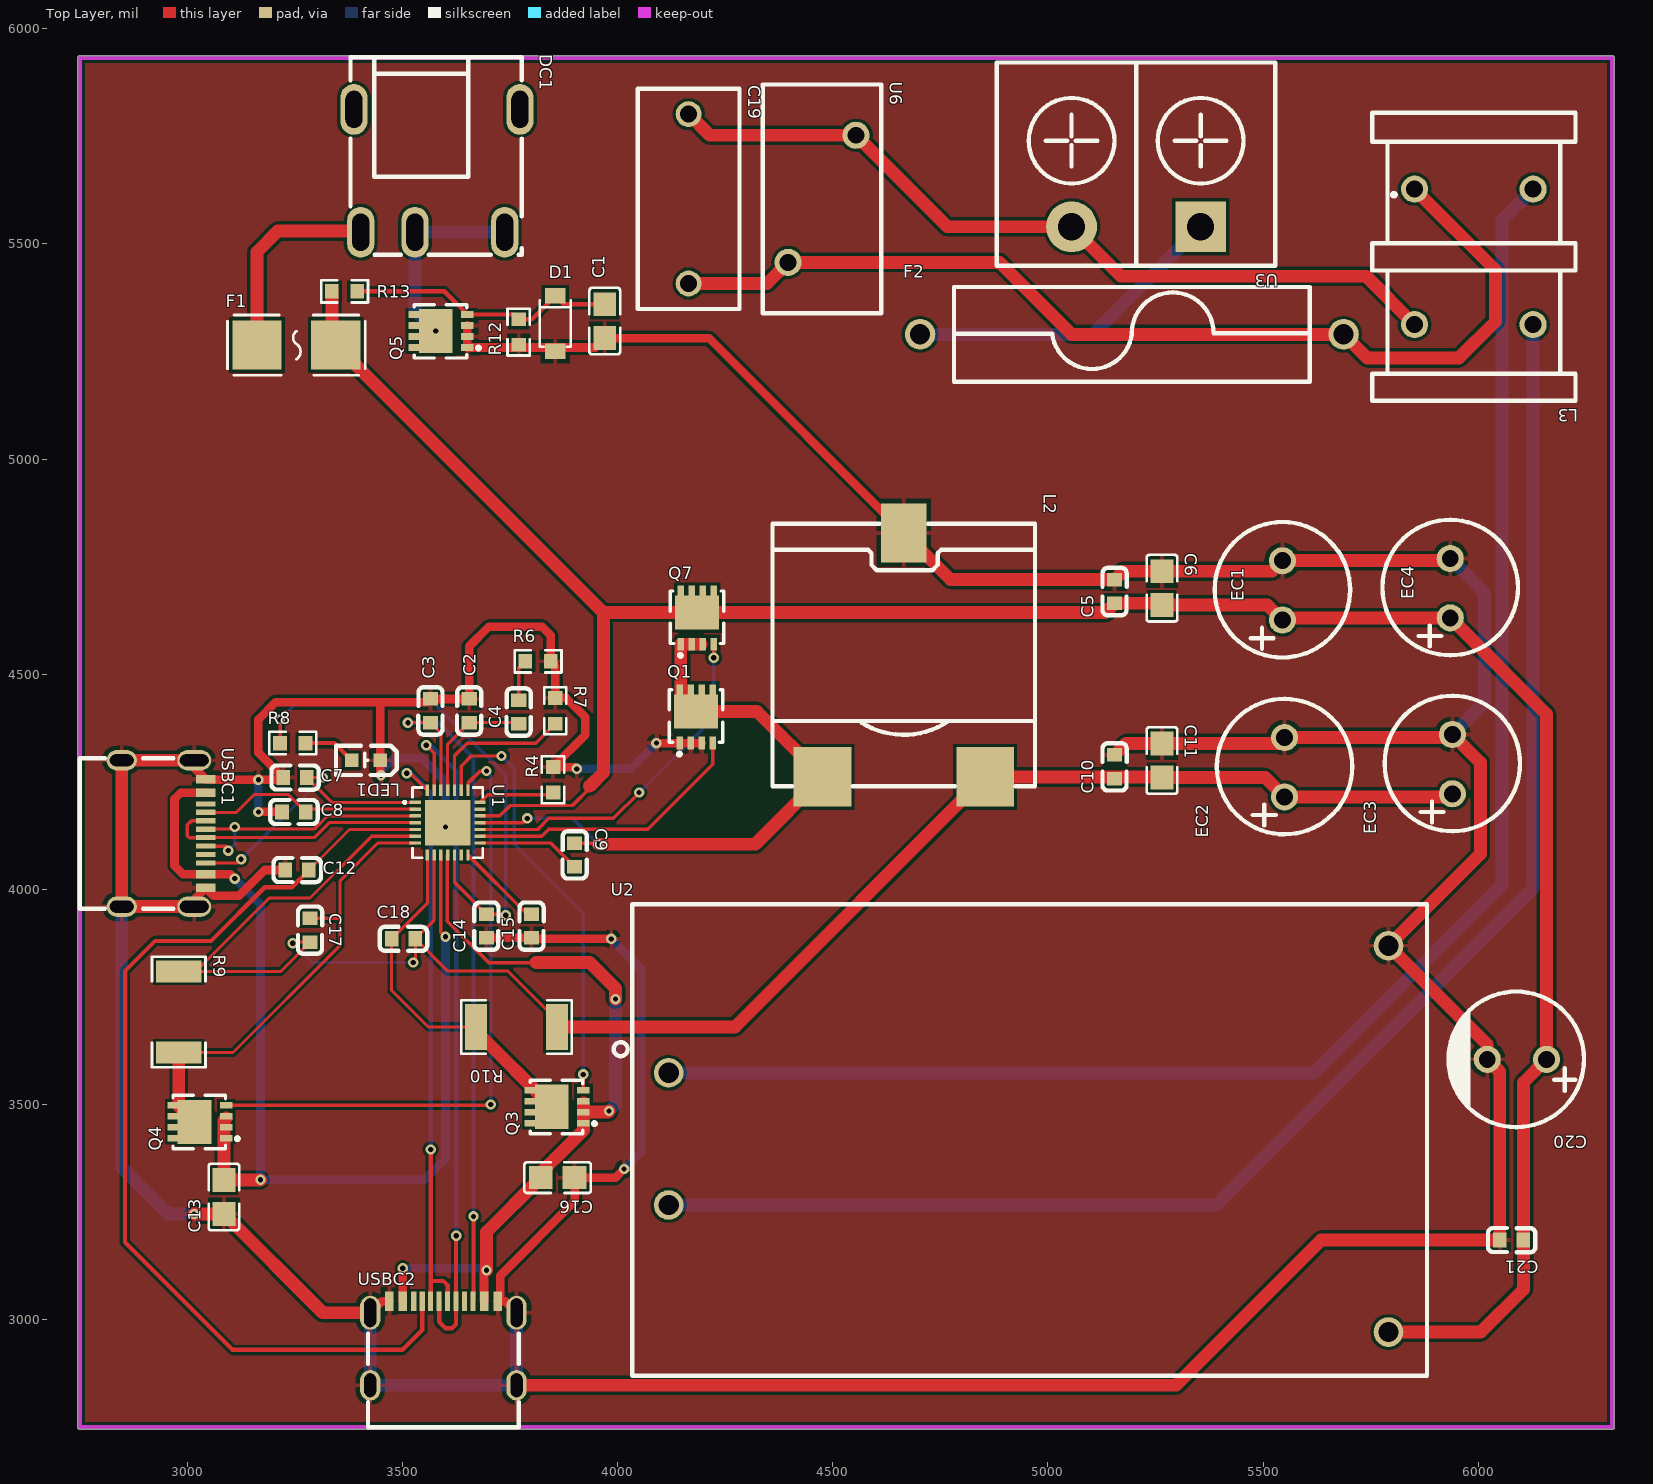
[diagram p0: Top Layer view]
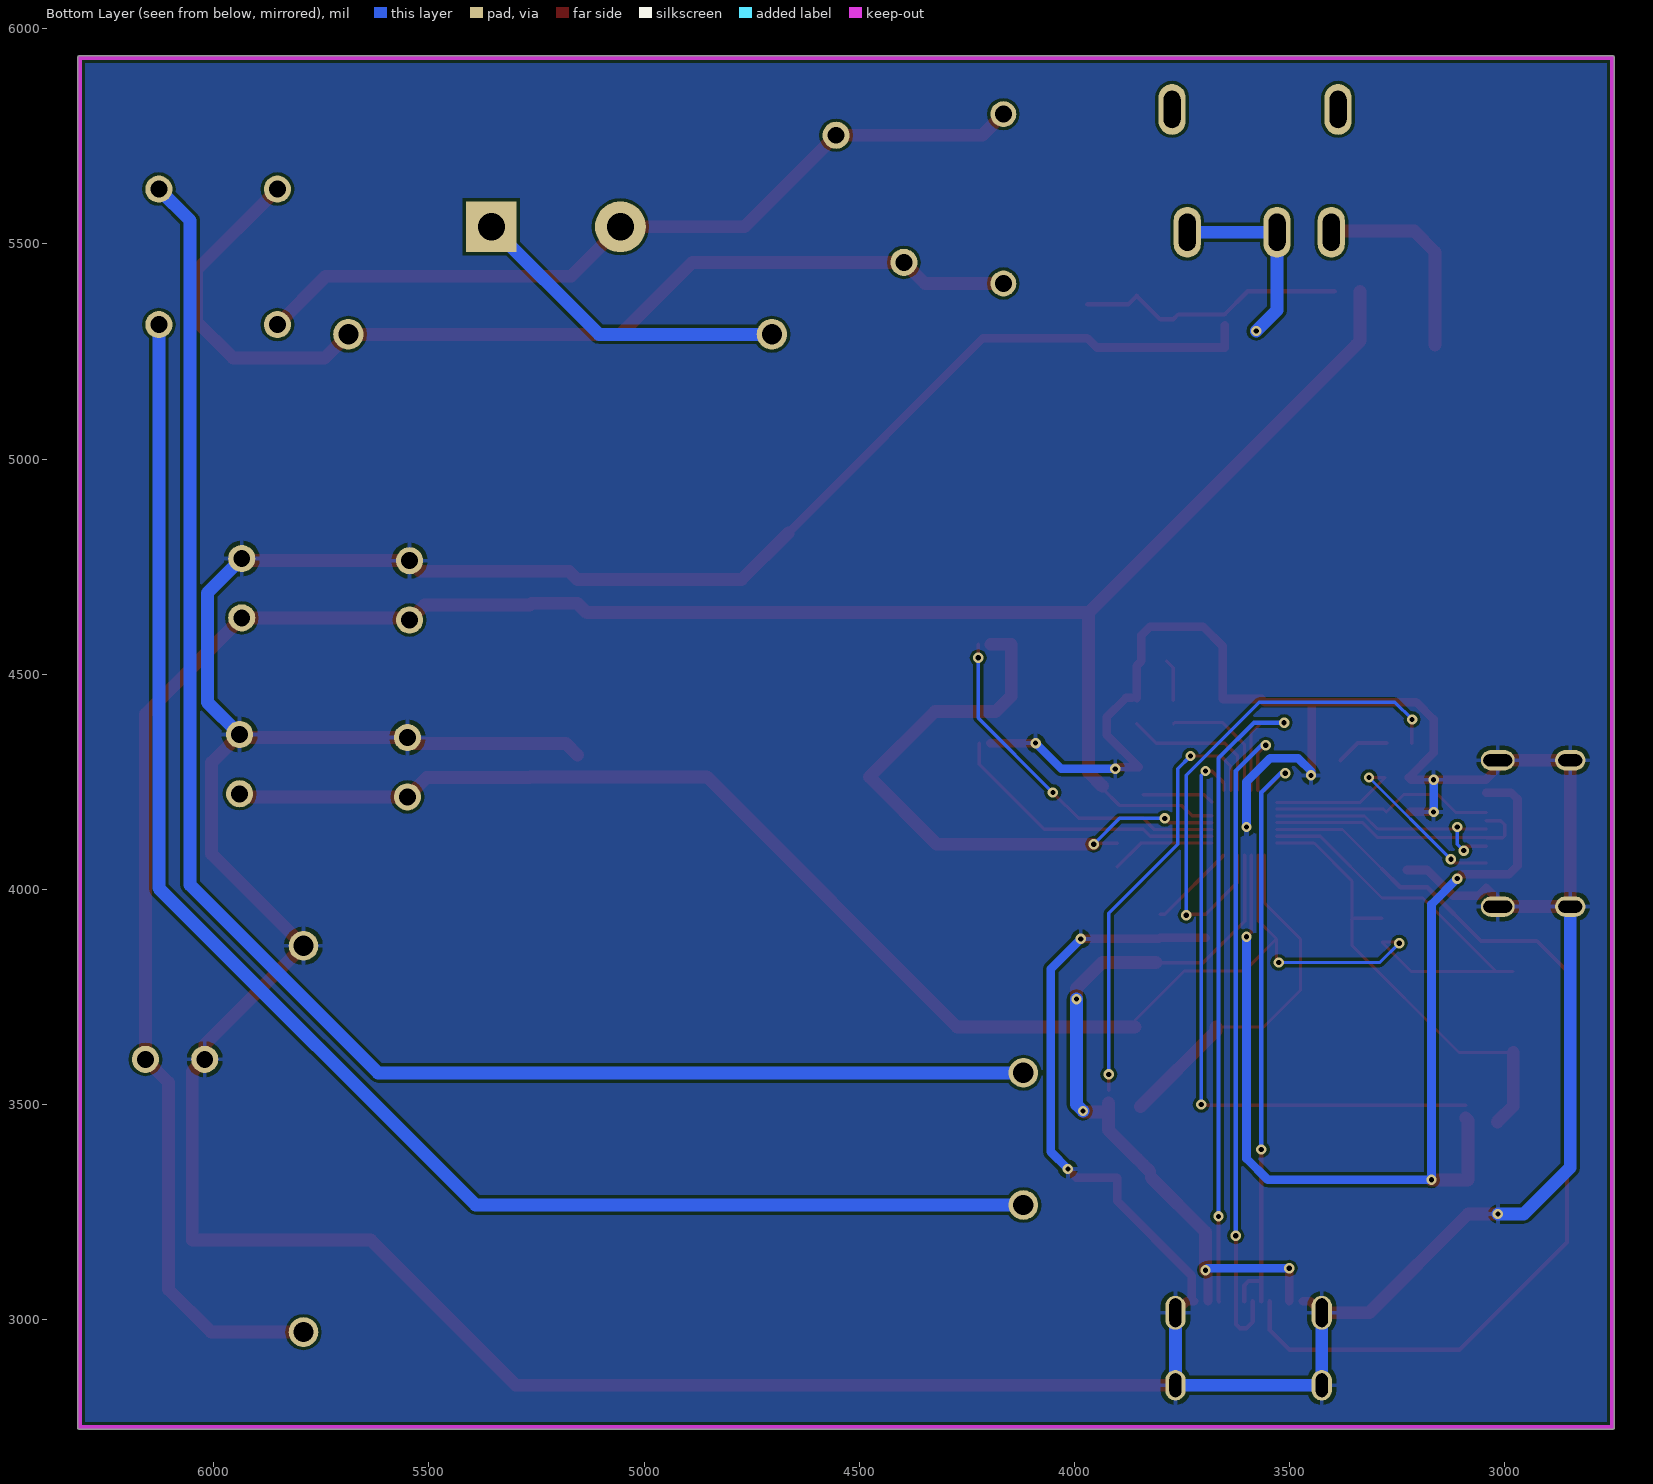
[diagram p1: Bottom Layer view, seen from below]
# Altium PCB MISC82101.pcbdoc
Units mil, origin at the board's own origin, x right, y up, seen from the top; angles counter-clockwise.
Board outline 3571.45 x 3192.71 mil, 2 copper layers (Top Layer, Bottom Layer); 51 components, 36 nets, 208 pads, 39 vias.

## Layer stack, top to bottom (the 12.6 mil dielectric is the usual default, probably not edited)
Top Solder Mask Layer: solder mask 0.4, Solder Resist, Dk 3.5
Top Layer: signal copper 1.4
Dielectric1: dielectric 12.6, FR-4, Dk 4.8
Bottom Layer: signal copper 1.4
Bottom Solder Mask Layer: solder mask 0.4, Solder Resist, Dk 3.5

## Board outline
2750,2744.99 cw(c2750,2750) 2744.99,2750 2744.99,5932.68 cw(c2750,5932.68) 2750,5937.69 6309.09,5937.69 cw(c6309.09,5932.68) 6310.26,5937.56 cw(c6311.42,5932.68) 6316.43,5932.68 6316.43,2750 cw(c6311.42,2750) 6311.42,2744.99

## Design rules (kind name [scope] priority, off if disabled: settings)
Clearance [All] p1: gap=7
MinimumSolderMaskSliver [All] p1: minsoldermaskwidth=0
PolygonConnect [All] p1: connectstyle=Relief reliefconductorwidth=10 reliefentries=4 polygonreliefangle="90 Angle" airgapwidth=10
RoutingVias [All] p1: holewidth=28 width=50 viastyle="Through Hole" minholewidth=28 minwidth=50 maxholewidth=28 maxwidth=50
SilkToSilkClearance [All] p1: silktosilkclearance=0
SilkToSolderMaskClearance [IsPad] p1: minsilkscreentomaskgap=0 clearancetoexposedcopper=TRUE
SolderMaskExpansion [All] p1: expansion=4
Width [All] p1: maxlimit=50 minlimit=7 preferedwidth=10 minimp=50.000000 maximp=50.000000 favimp=50.000000
27 further rules are at their usual default settings.

## Components (designator, comment, footprint, x,y, rotation, side; value= is the part's Value field where it differs from the comment)
C1 "10uF" C0805 3970,5320.63 r90 top
C2 "100pF" C0603 3655,4415 r90 top
C3 "330pF" C0603 3565,4415 r90 top
C4 "2.2nF" C0603 3770,4412.44 r90 top
C5 "100nF" C0603 5155,4692.56 r90 top
C6 "10uF" C0805 5265,4700 r270 top
C7 "330pF" C0603 3250,4260 r180 top
C8 "330pF" C0603 3247.44,4180 r180 top
C9 "100nF" C0603 3900,4080 r270 top
C10 "100nF" C0603 5155,4285 r90 top
C11 "22uF" C0805 5265,4299.37 r270 top
C12 "330pF" C0603 3255,4045 r180 top
C13 "10uF" C0805 3085,3285 r90 top
C14 "1uF" C0603 3695,3915 r90 top
C15 "1uF" C0603 3800,3915 r90 top
C16 "10uF" C0805 3860.63,3330 r180 top
C17 "100nF" C0603 3285,3905 r270 top
C18 "100nF" C0603 3502.44,3885 r0 top
C19 "100nF" CAP-TH_L13.0-W6.0-P10.0-D0.6 4165,5605 r270 top
C20 "220uF" CAP-TH_BD8.0-P3.50-D0.6-FD 6090,3605 r180 top
C21 "100nF" C0603 6077.56,3185 r180 top
D1 "BZT52C3V3" SOD-123_L2.7-W1.6-LS3.7-RD 3855,5315 r270 top
DC1 "DC-044A-20A" DC-IN-TH_DC-044A-20A 3580,5670 r270 top
EC1 "220uF" CAP-TH_BD8.0-P3.50-D0.6-FD-2 5545,4695 r90 top
EC2 "220uF" CAP-TH_BD8.0-P3.50-D0.6-FD-2 5550,4283.9 r90 top
EC3 "220uF" CAP-TH_BD8.0-P3.50-D0.6-FD-2 5940,4291.1 r90 top
EC4 "220uF" CAP-TH_BD8.0-P3.50-D0.6-FD-2 5935,4700 r90 top
F1 "0451008.MRL" FUSE-SMD_L6.1-W2.7 3253.3,5265 r0 top
F2 "5G.0015222000S1(5)" FUSE-TH_BD5.6-L21.0-P25.00-D0.7 5195,5290 r0 top
L2 "22uH" IND-SMD_3P-L15.5-W15.5-L 4665,4545 r270 top
L3 "UU9.8-20mH" FILTER-TH_4P-L17.0-W12.0-P7.00-D0.6-S8.00 5990,5470 r180 top
LED1 "19-217/BHC-ZL1M2RY/3T" LED0603-R-RD 3415,4300 r180 top
Q1 "RUH4040M2" PDFN3333-8_L3.1-W3.2-P0.65-LS3.4-BL 4182.79,4400.37 r0 top
Q3 "RUH4040M2" PDFN3333-8_L3.1-W3.2-P0.65-LS3.4-BL 3860,3495 r90 top
Q4 "RUH4040M2" PDFN3333-8_L3.1-W3.2-P0.65-LS3.4-BL 3030,3460 r90 top
Q5 "RUH4040M2" PDFN3333-8_L3.1-W3.2-P0.65-LS3.4-BL 3590.37,5297.79 r90 top
Q7 "RUH4040M2" PDFN3333-8_L3.1-W3.2-P0.65-LS3.4-BL 4185,4630 r0 top
R4 "Rpset" R0603 3850,4254.66 r270 top
R6 "20kΩ" R0603 3815,4530 r0 top
R7 "SDNT1608X104F4250FTF" R0603 3855,4415 r270 top
R8 "0603WAF2001T5E" R0603 3245,4340 r0 top
R9 "RLM20FECR005" R2010 2980,3715 r270 top
R10 "RLM20FECR005" R2010 3765,3680 r180 top
R12 "10kΩ" R0603 3770,5295.34 r90 top
R13 "0603WAF5102T5E" R0603 3365.34,5390 r180 top
U1 "sw3556-1" QFN-28_L4.0-W4.0-P0.40-BL-EP 3605,4155 r270 top
U2 "HLK-10M24" PWRM-TH_HLK-10M24 4955,3420 r0 top
U3 "KF7.62-2P" CONN-TH_KF7.62-2P 5205,5540 r180 top
U6 "10D561K68RV0095" RES-TH_L13.5-W7.0-P7.50-S4.00-D0.7 4475,5605 r270 top
USBC1 "U263-163N-4OS1735" USB-C-SMD_U263-163N-4GS1735 2945,4130 r270 top
USBC2 "U263-163N-4OS1735" USB-C-SMD_U263-163N-4GS1735 3595,2945 r0 top

## Footprints (in the part's own frame and the unit in brackets; to place one, negate y for a bottom-side part, rotate by r counter-clockwise, add the part's x,y. Pads: shape width x height; smd on the part's side, far side on the other; paste and mask are expansions set on the pad)
C0603 [mm]
  rect 0.8x0.9 smd paste+0 mask+0.051: 1(-0.7,0) 2(0.7,0)
  silkscreen extent -1.41,-0.71 1.39,0.72
C0805 [mm]
  rect 1.41x1.35 smd paste-100 mask+0.051: 1(-1,0) 2(1,0)
  silkscreen extent -1.96,-0.9 1.96,0.9
CAP-TH_BD8.0-P3.50-D0.6-FD [mm]
  round 1.6 hole 1: 1(-1.75,0) 2(1.75,0)
  silkscreen extent -3.96,-4 4.04,4
CAP-TH_BD8.0-P3.50-D0.6-FD-2 [mm]
  round 1.6 hole 1 paste+0 mask+0.051: 1(-1.75,0) 2(1.75,0)
  silkscreen extent -3.96,-4 4.04,4
CAP-TH_L13.0-W6.0-P10.0-D0.6 [mil]
  round 60 hole 39.37: 1(-196.85,0) 2(196.85,0)
  silkscreen extent -256,-118 256,118
CONN-TH_KF7.62-2P [mm]
  rect 3x3 hole 1.6: 1(-3.81,0)
  round 3 hole 1.6: 2(3.81,0)
  silkscreen extent -8.22,-9.7 8.22,2.3
DC-IN-TH_DC-044A-20A [mm]
  oval 3x1.6 hole 1 slot 2.2 at 0 deg paste+0 mask+0.051: 1(3.625,-4.5) 2(3.625,4.001) 3(3.625,-1.3) 4(-3.625,-4.9) 5(-3.625,4.9)
  silkscreen extent -6.7,-5.1 4.95,5
FILTER-TH_4P-L17.0-W12.0-P7.00-D0.6-S8.00 [mm]
  round 1.6 hole 1: 1(3.5,-4) 2(-3.5,-4) 3(-3.5,4) 4(3.5,4)
  silkscreen extent -6,-8.5 6,8.5
FUSE-SMD_L6.1-W2.7 [mil]
  rect 114.6x114.4 smd paste-3937.01 mask+2: 1(-91.7,0) 2(91.7,0)
  silkscreen extent -160,-70 160,70
FUSE-TH_BD5.6-L21.0-P25.00-D0.7 [mm]
  round 1.8 hole 1.2: 1(-12.5,0) 2(12.5,0)
  silkscreen extent -10.5,-2.8 10.5,2.8
IND-SMD_3P-L15.5-W15.5-L [mil]
  rect 137.8x106.3 smd paste+0 mask+2: 1(-283.5,0)
  rect 137.8x133.9 smd paste+0 mask+2: 2(283.5,-189) 3(283.5,189)
  silkscreen extent -305,-305 305,305
LED0603-R-RD [mm]
  rect 0.8x0.8 smd paste+0 mask+0.051: 1(0.851,0) 2(-0.851,0)
  silkscreen extent -1.82,-0.86 1.77,0.86
PDFN3333-8_L3.1-W3.2-P0.65-LS3.4-BL [mm]
  rect 0.4x0.75 smd paste-100 mask+0.051: 1(-0.975,-1.533) 2(-0.325,-1.533) 3(0.325,-1.533) 4(0.975,-1.533)
  rect 0.4x0.8 smd paste-100 mask+0.051: 5(0.975,1.533) 6(0.325,1.533) 7(-0.325,1.533) 8(-0.975,1.533)
  rect 2.6x2 smd paste-100 mask+0.051: 9(-0.005,0.333)
  silkscreen extent -1.59,-2.29 1.56,1.61
PWRM-TH_HLK-10M24 [mm]
  round 1.75 hole 1.2 paste+0 mask+0.05: 1(-21.25,3.9) 2(-21.25,-3.9) 3(21.25,11.4)
  round 1.75 hole 1.2 copper offset 0,0 paste+0 mask+0.05: 4(21.25,-11.4)
  silkscreen extent -24.49,-13.98 23.52,13.86
QFN-28_L4.0-W4.0-P0.40-BL-EP [mm]
  rect 0.2x0.665 smd paste-100 mask+0.051: 1(-1.2,-1.908) 2(-0.8,-1.908) 3(-0.4,-1.908) 4(0,-1.908) 5(0.4,-1.908) 6(0.8,-1.908) 7(1.2,-1.908) 15(1.2,1.908) 16(0.8,1.908) 17(0.4,1.908) 18(0,1.908) 19(-0.4,1.908) 20(-0.8,1.908) 21(-1.2,1.908)
  rect 0.665x0.2 smd paste-100 mask+0.051: 8(1.908,-1.2) 9(1.908,-0.8) 10(1.908,-0.4) 11(1.908,0) 12(1.908,0.4) 13(1.908,0.8) 14(1.908,1.2) 22(-1.908,1.2) 23(-1.908,0.8) 24(-1.908,0.4) 25(-1.908,0) 26(-1.908,-0.4) 27(-1.908,-0.8) 28(-1.908,-1.2)
  rect 2.7x2.7 smd paste-100 mask+0.051: 29(0,0)
  silkscreen extent -2.08,-2.61 2.08,2.08
R0603 [mil]
  rect 31.75x34.02 smd paste-3937.01 mask+2: 1(-29.66,0) 2(29.66,0)
  silkscreen extent -55,-26 55,26
R2010 [mm]
  rect 1.283x2.7 smd paste-100 mask+0.051: 1(-2.391,0) 2(2.391,0)
  silkscreen extent -3.26,-1.58 3.26,1.58
RES-TH_L13.5-W7.0-P7.50-S4.00-D0.7 [mm]
  round 1.6 hole 1 paste+0 mask+0.05: 1(-3.75,2) 2(3.75,-2)
  silkscreen extent -6.75,-3.5 6.75,3.5
SOD-123_L2.7-W1.6-LS3.7-RD [mm]
  rect 0.91x1.22 smd paste+0 mask+0.051: 1(-1.635,0) 2(1.635,0)
  silkscreen extent -1.38,-0.93 1.38,0.93
USB-C-SMD_U263-163N-4GS1735 [mm]
  rect 0.5x1.15 smd paste-100 mask+0.051: A1(-3.2,2.478) A4(-2.4,2.478) A9(2.4,2.478) A12(3.218,2.478) B1(3.218,2.478) B4(2.4,2.478) B9(-2.4,2.478) B12(-3.2,2.478)
  rect 0.3x1.15 smd paste-100 mask+0.051: A5(-1.25,2.478) A6(-0.25,2.478) A7(0.25,2.478) A8(1.25,2.478) B5(1.75,2.478) B6(0.75,2.478) B7(-0.75,2.478) B8(-1.75,2.478)
  oval 1.2x1.8 hole 0.7 slot 1.4 at 90 deg paste+0 mask+0.051: SH1(-4.32,-2.477) SH1(4.32,-2.477)
  oval 1.2x2 hole 0.7 slot 1.7 at 90 deg copper offset 0,0 paste+0 mask+0.051: SH1(-4.32,1.802)
  oval 1.2x2 hole 0.7 slot 1.7 at 90 deg paste+0 mask+0.051: SH1(4.32,1.802)
  silkscreen extent -4.44,-4.96 4.45,0.58

## Part data
C1 C6 C13 C16: "Capacitance: 10uF; tolerance: ±10%; rated voltage: 50V; dielectric (temperature coefficient): X5R;"
C2: "Capacitance: 100pF; tolerance: ±5%; rated voltage: 50V; dielectric (temperature coefficient): C0G;"
C3 C7 C8 C12: "Capacitance: 330pF; tolerance: ±5%; rated voltage: 50V; dielectric (temperature coefficient): C0G;"
C4: "Capacitance: 2.2nF; tolerance: ±1%; rated voltage: -; dielectric (temperature coefficient): -;"
C5 C9 C10 C17 C18 C21: "Capacitance: 100nF; tolerance: ±10%; rated voltage: 50V; dielectric (temperature coefficient): X7R;"
C11: "Capacitance: 22uF; tolerance: ±20%; rated voltage: 25V; dielectric (temperature coefficient): X5R;"
C14 C15: "Capacitance: 1uF; tolerance: ±10%; rated voltage: 50V; dielectric (temperature coefficient): X5R;"
C19: library part X2-104K-275VAC_C914483
C20: library part 01EC3470
D1: "Diode configuration: single; zener voltage (nominal): 3.3V; zener voltage (range): 3.1V~3.5V; tolerance: ±5%; power: 500mW; reverse current (Ir): 20uA@1V; impedance (Zzt): 130Ω;"
DC1: "Contact inner diameter: 2mm; contact outer diameter: 5.9mm; rated current: 500mA; rated voltage: 30V;"
EC1 EC2 EC3 EC4: "容值:220uF;精度:±20%;额定电压:35V;电容体直径:8mm;电容体长度:9mm;脚间距:3.5mm;纹波电流:1.7A@100kHz;等效串联电阻:40mΩ@100kHz;工作寿命:2000hrs@105℃;工作温度:-55℃~+105℃;"
F1: "Type: SMD fuse; rated current: 8A; rated voltage (AC): 125V; rated voltage (DC): 125V; breaking capacity: 50A; operating temperature: -55℃~+125℃;"
L2: "Inductance: 22uH; tolerance: ±20%; rated current: 7.5A; DC resistance (DCR): 14.5mΩ;"
LED1: "Illumination color: blue; dominant wavelength / chromaticity: 465~475nm;"
Q1 Q3 Q4 Q5 Q7: "类型:-;漏源电压(Vdss):-;连续漏极电流(Id):-;功率(Pd):-;导通电阻(RDS(on)@Vgs,Id):-;阈值电压(Vgs(th)@Id):-;栅极电荷(Qg@Vgs):-;输入电容(Ciss@Vds):-;反向传输电容(Crss@Vds):-;"
R4: "Resistor"
R6: "Tolerance: ±1%; temperature coefficient: ±100ppm/℃; resistance: 20kΩ; power: 1/10W; max working voltage: 75V; operating temperature range: -55℃~+155℃;"
R7: "阻值(25℃):100kΩ;电阻精度:±1%;B值精度:±1%;B值(25℃/50℃):4250K;功率:100mW;最大稳态电流(25℃):100uA;B值(25℃/75℃):-;B值(25℃/85℃):-;B值(25℃/100℃):-;工作温度:-55℃~+125℃;"
R8: "Tolerance: ±1%; resistance: 2kΩ; temperature coefficient: ±100ppm/℃; power: 1/10W; max working voltage: 75V; operating temperature range: -55℃~+155℃;"
R9 R10: "Resistor type: sense resistor; rated current: -; rated voltage drop: -; resistance: 5mΩ; tolerance: ±1%; power: 1W; temperature coefficient: ±50ppm/℃; mounting: SMD;"
R12: "Resistor type: thick film; resistance: 10kΩ; tolerance: ±1%; power: 100mW; temperature coefficient: ±100ppm/℃; max working voltage: 75V; operating temperature range: -55℃~+155℃;"
USBC1 USBC2: "连接器类型:Type-C;标准:USB 3.1;公母:母座;触点数量:16;端口数量:1;安装方式:卧贴;额定电流 - 电源:5A;触头材质:铜合金;触头镀层:金;工作温度范围:-25℃~+85℃;焊接温度(最大值):260℃;"

## Via types
v1: diameter 24, hole 12, Top Layer to Bottom Layer, 39 vias

## Nets (pads, with @x,y where several pads share a name; then routed paths per layer and width w, separated by ;. In a path a pad name is that pad's centre, name@x,y a point inside that pad or via, vN(x,y) a via of type N, cw(c..) or ccw(c..) an arc to the next point about the centre after c; other vN are vias at no path point)
BST: C9.2 U1.15 | length 242.8
  Top Layer w8: U1.15 3844.68,4107.76 C9.2
CC11: C8.1 U1.2 USBC1.A5 | length 523.5
  Top Layer w7: USBC1.A5 3114.21,4179.21 3155,4220 3235,4220 C8.1 3281.5,4186.5 U1.2
CC12: C12.1 U1.5 USBC2.A5 | length 2321.3
  Top Layer w7: C12.1@3285,4047.44 3376.81,4139.25 U1.5
  Top Layer w10: C12.1@3285,4047.44 C12.1 3242.56,4005 3180,4005 3055,3880 2925,3880 2855,3810 2855,3180 3105,2930 3500,2930 3545.79,2975.79 USBC2.A5
CC21: C7.1 U1.1 USBC1.B5 | length 668.6
  Top Layer w7: USBC1.B5 3116.1,4061.1 v1(3125,4070) ; v1(3315,4260) C7.1 3335.32,4202.24 U1.1
  Bottom Layer w7: v1(3125,4070) v1(3315,4260)
CC22: C3.1 U1.26 USBC2.B5 | length 1673
  Top Layer w7: v1@3510,4385 v1(3512.44,4387.44) C3.1 3589.25,4363.19 U1.26
  Top Layer w10: USBC2.B5 3665,3043.64 v1(3665,3240)
  Bottom Layer w10: v1(3512.44,4387.44) 3582.56,4387.44 3665,4305 v1(3665,3240)
COMP: C2.1 C4.1 U1.25 | length 294.1
  Top Layer w7: U1.25 3605,4337.44 C2.1 3767.44,4387.44 C4.1
CSN1: C17.1 Q4.5 Q4.6 Q4.7 Q4.8 Q4.9 R9.2 U1.7 | length 1086.8
  Top Layer w7: R9.2 3105.86,3620.86 3355,3870 3355,3930 3355,4020 3442.76,4107.76 U1.7
  Top Layer w8: C17.1 3352.44,3932.56 3355,3930
  Top Layer w30: R9.2 2980,3496.71 Q4.9
CSN2: C18.1 Q3.5 Q3.6 Q3.7 Q3.8 Q3.9 R10.2 U1.8 | length 838.4
  Top Layer w7: U1.8 3557.76,3967.88 C18.1 3474.88,3765.12 3560,3680 R10.2
  Top Layer w30: R10.2 3670.86,3670.85 Q3.9
CSP1: C10.1 C11.2 C17.2 C18.2 EC2.1 EC3.1 L2.3 R9.1 R10.1 U1.6 U1.9 | length 4351.2
  Top Layer w7: R9.1 R9.1@3019.14,3809.14 ; v1(3245,3875) 3247.44,3877.44 C17.2 3216.7,3809.14 R9.1@3019.14,3809.14 ; v1(3525,3830) 3530,3835 C18.2 ; U1.6 3428.5,4123.5 3285,3980 3190,3980 R9.1@3019.14,3809.14 ; U1.9 3573.5,3928.5 C18.2 ; R10.1 3859.14,3695.86 3745,3810 3605,3810 C18.2
  Top Layer w30: R10.1 4272.5,3680 L2.3 5263.5,4261.5 C11.2 5505,4260 EC2.1 5932.8,4215 EC3.1
  Bottom Layer w7: v1(3245,3875) 3290,3830 v1(3525,3830)
DM1: U1.4 USBC1.A7 USBC1.B7 | length 618
  Top Layer w7: USBC1.A7 3294.95,4120.15 3329.8,4155 U1.4
  Top Layer w8: USBC1.A7 3005.15,4120.15 3005,4120 3000,4125 3000,4150 3009.52,4159.52 USBC1.B7
DM2: U1.28 USBC2.A7 USBC2.B7 | length 1402.2
  Top Layer w8: v1(3510,4270) 3517.86,4270 U1.28
  Top Layer w10: USBC2.B7 3565.48,3090 ; v1(3565.48,3395.48) 3565.48,3090 ; USBC2.A7 3604.85,3080.15 3595,3090 3565.48,3090
  Bottom Layer w10: v1(3510,4270) 3520.96,4270 3565.48,4225.48 v1(3565.48,3395.48)
DP1: U1.3 USBC1.A6 USBC1.B6 | length 613.4
  Top Layer w7: USBC1.A6 3294.84,4139.84 3325.75,4170.75 U1.3
  Top Layer w8: USBC1.B6 v1@3089.53,4100.47 ; v1@3095,4085 v1(3095,4090)
  Bottom Layer w8: v1(3095,4090) 3110,4105 v1(3110,4145)
DP2: U1.27 USBC2.A6 USBC2.B6 | length 1590.2
  Top Layer w8: v1(3555,4335) 3573.5,4316.5 U1.27
  Top Layer w10: USBC2.A6 3585.16,2994.84 3600,2980 3615,2980 3624.53,2989.53 USBC2.B6 3624.53,3194.53 v1(3625,3195)
  Bottom Layer w10: v1(3555,4335) 3565,4335 3625,4275 v1(3625,3195)
GATE1: Q4.4 U1.22 | length 1465.8
  Top Layer w8: Q4.4 3703.39,3498.39 v1(3705,3500) ; U1.22 3652.24,4247.24 3680,4275 v1(3695,4275)
  Bottom Layer w8: v1(3695,4275) 3705,4265 v1(3705,3500)
GATE2: Q3.4 U1.23 | length 1015.1
  Top Layer w8: U1.23 3636.5,4286.5 3660,4310 v1(3730,4310) ; v1(3920,3570) 3920.37,3569.63 Q3.4
  Bottom Layer w8: v1(3730,4310) 3760,4280 3760,4105 3920,3945 v1(3920,3570)
GND: C1.1 C2.2 C3.2 C5.2 C6.1 C7.2 C8.2 C10.2 C11.1 C12.2 C13.1 C14.1 C15.1 C16.1 C20.2 C21.2 D1.2 EC1.2 EC2.2 EC3.2 EC4.2 L2.1 LED1.2 Q1.1 Q1.2 Q1.3 Q5.1 Q5.2 Q5.3 R4.1 R6.2 R7.1 R12.1 U1.29 U2.3 USBC1.A1 USBC1.A12 USBC1.B1 USBC1.B12 USBC1.SH1 USBC2.A1 USBC2.A12 USBC2.B1 USBC2.B12 USBC2.SH1 | length 14705.9
  Top Layer w20: USBC1.SH1@3015.96,3959.92 3015.96,3976.7 USBC1.B1 3060.83,3985 3120,3985 3180,4045 C12.2 ; USBC1.SH1@3015.96,4300.07 3015.96,4282.57 USBC1.B12 3043.52,4255 v1(3165,4255) 3217.44,4255 C7.2 3165,4317.44 3165,4395 3205,4435 3450,4435 ; v1(3165,4180) C8.2 ; USBC2.SH1@3424.93,3015.96 3451.51,3042.54 USBC2.B12 ; v1(3450,4265) 3448.5,4266.5 LED1.2 3448.5,4433.5 3450,4435 ; Q5.3 Q5.2 Q5.1 3948.14,5259.4 C1.1 4212.24,5281.26 L2.1 ; C14.1 C15.1 3802.44,3885 v1(3985,3885) ; USBC2.SH1@3765.08,3015.96 3738.5,3042.54 USBC2.B1 3727,3047.83 3727,3102 3900,3275 C16.1 3995,3330 v1(4015,3350) ; R7.1 3855,4519.66 R6.2 3844.66,4590.34 3825,4610 3700,4610 3655,4565 C2.2 C3.2 3557.44,4435 3450,4435 ; R7.1@3865,4445 3880,4445 3925,4400 3925,4359.32 R4.1 3900.68,4284.32 v1(3905,4280) ; v1(4090,4340) Q1.1 Q1.2 Q1.3
  Top Layer w30: USBC1.SH1@2847.47,4300.07 USBC1.SH1@3015.96,4300.07 ; USBC1.SH1@2847.46,4300.08 2847.46,3959.92 USBC1.SH1@3015.95,3959.92 ; v1(3015.63,3245.63) C13.1 3314.67,3015.96 USBC2.SH1@3424.93,3015.96 ; USBC2.SH1@3765.08,2847.46 5297.46,2847.46 5635,3185 C21.2 6050,3576.1 C20.2 6021.1,3639.32 U2.3 6005,4082.21 6005,4295 EC3.2 5932.8,4352.8 EC2.2 5535.94,4338.74 C11.1 5181.18,4338.74 C10.2 ; L2.1 4773.38,4720.12 C5.2 5174.25,4739.37 C6.1 5520.47,4739.37 EC1.2 5930,4763.9 EC4.2
  Bottom Layer w20: v1(3165,4180) v1(3165,4255) ; v1(3450,4265) 3450,4275 3480,4305 3545,4305 3600,4250 v1(3600,4145) ; v1(3905,4280) 4030,4280 v1(4090,4340) ; v1(3985,3885) 4055,3815 4055,3390 v1(4015,3350)
  Bottom Layer w30: USBC1.SH1@2847.46,3959.92 2847.46,3353.8 2955.63,3245.63 v1(3015.63,3245.63) ; USBC2.SH1@3424.92,2847.46 3765.08,2847.46 USBC2.SH1@3765.08,3015.96 ; USBC2.SH1@3424.93,2847.47 USBC2.SH1@3424.93,3015.96 ; EC4.2 6015,4688.91 6015,4435 EC3.2
HGATE: Q7.4 U1.17 | length 826.7
  Top Layer w8: U1.17 3814.25,4139.25 3840,4165 3990,4165 v1(4050,4225) ; v1@4220,4535 v1(4223.39,4538.39) Q7.4
  Bottom Layer w8: v1(4050,4225) 4223.39,4398.39 v1(4223.39,4538.39)
LGATE: Q1.4 U1.16 | length 659.4
  Top Layer w8: U1.16 3823.5,4123.5 3840,4140 4070,4140 4221.18,4291.18 Q1.4
NetC1_2: C1.2 D1.1 Q5.4 R12.2 R13.1 | length 632.5
  Top Layer w10: R13.1 3596.92,5390 Q5.4 3758.82,5336.18 R12.2 3800.63,5325 D1.1 3874.37,5360 C1.2
NetC4_2: C4.2 R6.1 | length 96.4
  Top Layer w8: C4.2 3770,4514.66 R6.1
NetC15_2: C15.2 U1.14 | length 204.6
  Top Layer w8: U1.14 3789.58,3942.56 C15.2
NetC19_1: C19.1 L3.4 U3.2 U6.1 | length 1889.9
  Top Layer w30: C19.1 4214.21,5752.64 U6.1 4766.38,5540 U3.2 5170,5425 5739.72,5425 L3.4
NetC19_2: C19.2 F2.2 L3.1 U6.2 | length 2408
  Top Layer w30: C19.2 4347.05,5408.15 U6.2 4887.64,5457.36 5055,5290 F2.2 5742.13,5235 5955,5235 6040,5320 6040,5439.68 L3.1
NetDC1_1: DC1.1 F1.1 | length 479
  Top Layer w30: F1.1 3161.6,5481.6 3210,5530 3400.1,5530 DC1.1
NetDC1_2: DC1.2 DC1.3 Q5.5 Q5.6 Q5.7 Q5.8 Q5.9 | length 458.4
  Bottom Layer w30: v1(3577.26,5297.61) 3528.82,5346.06 DC1.3 DC1.2
NetF2_1: F2.1 U3.1 | length 755.7
  Bottom Layer w30: F2.1 5105,5290 U3.1
NetL3_2: L3.2 U2.1 | length 3765
  Bottom Layer w30: U2.1 5618.55,3573.55 6055,4010 6055,5554.68 L3.2
NetL3_3: L3.3 U2.2 | length 3624.1
  Bottom Layer w30: U2.2 5391.45,3266.45 6127.8,4002.8 L3.3
NetLED1_1: LED1.1 R8.2 | length 123.4
  Top Layer w10: R8.2 3341.5,4340 LED1.1
NetR4_2: R4.2 U1.21 | length 167.3
  Top Layer w8: U1.21 3697.86,4220 R4.2@3840,4220
NTC: R7.2 U1.24 | length 345.8
  Top Layer w8: U1.24 3620.75,4310.75 3650,4340 3809.66,4340 R7.2
SW: C9.1 L2.2 Q1.5 Q1.6 Q1.7 Q1.8 Q1.9 Q7.1 Q7.2 Q7.3 U1.18 | length 1524.4
  Top Layer w7: Q7.3@4193.52,4569.63 Q7.3
  Top Layer w8: U1.18 3780,4155 v1(3790,4165) ; C9.1 3952.44,4107.56 v1(3955,4105)
  Top Layer w30: v1(3955,4105) 4319.5,4105 L2.2 4324.02,4413.48 Q1.9 4146.61,4449.48 Q7.1 Q7.2 Q7.3@4193.52,4569.63
  Bottom Layer w8: v1(3790,4165) 3895,4165 v1(3955,4105)
VBUS1: C13.2 Q4.1 Q4.2 Q4.3 U1.10 USBC1.A4 USBC1.A9 USBC1.B4 USBC1.B9 | length 2503.2
  Top Layer w8: U1.10 3589.25,3900.75 v1(3600,3890)
  Top Layer w20: USBC1.B9 3042.02,4225 2985,4225 2970,4210 2970,4055 2989.49,4035.51 USBC1.B4 3099.49,4035.51 v1(3110,4025)
  Top Layer w30: Q4.3@3090.37,3468.52 3085,3463.15 C13.2 3169.37,3324.37 v1(3170,3325)
  Bottom Layer w20: v1(3110,4025) 3170,3965 v1(3170,3325) 3550.48,3325 3600,3374.52 v1(3600,3890)
VBUS2: C16.2 Q3.1 Q3.2 Q3.3 U1.11 USBC2.A4 USBC2.A9 USBC2.B4 USBC2.B9 | length 1776.1
  Top Layer w8: U1.11 3604.25,4079.15 3604.25,3925.75 3700,3830 3810,3830
  Top Layer w20: v1@3500,3120 v1(3500.52,3119.48) USBC2.B9 ; USBC2.B4 3689.49,3109.49 v1(3695,3115)
  Top Layer w30: v1(3695,3115) 3695,3203.74 C16.2 ; 3810,3830 3935,3830 3995,3770 v1(3995,3745) ; C16.2@3825,3345 3840.24,3360.24 3840.24,3360.69 3853.13,3373.57 3853.57,3373.57 3920.37,3440.37 Q3.1 Q3.2 ; Q3.3@3920.37,3503.52 Q3.2 ; v1(3980,3485) 3977.21,3482.21 Q3.2
  Bottom Layer w20: v1(3500.52,3119.48) 3690.52,3119.48 v1(3695,3115)
  Bottom Layer w30: v1(3980,3485) 3995,3500 v1(3995,3745)
VDD: C14.2 R8.1 U1.12 | length 1206.3
  Top Layer w8: v1(3215,4395) 3215.34,4394.66 R8.1 ; U1.12 3620.75,4016.81 C14.2 3737.44,3942.56 v1(3740,3940)
  Bottom Layer w8: v1(3215,4395) 3255,4435 3570,4435 3740,4265 v1(3740,3940)
VIN: C5.1 C6.2 C20.1 C21.1 EC1.1 EC4.1 F1.2 Q7.5 Q7.6 Q7.7 Q7.8 Q7.9 R13.2 U1.19 U2.4 | length 5737
  Top Layer w8: U1.19 3725.75,4170.75 3750,4195 3895,4195 3935,4235 3935,4240
  Top Layer w30: R13.2 3335.68,5274.32 F1.2 3966.89,4643.11 ; 3935,4240 3966.89,4271.89 3966.89,4643.11 ; U2.4 6006.17,2971.17 6105.12,3070.12 C21.1 6105.12,3551.22 C20.1 6158.9,4407.21 EC4.1 5550,4631.1 EC1.1 5510.48,4660.63 C6.2 5260.63,4665 C5.1 5133.11,4643.11 Q7.9 3966.89,4643.11
pads on no net: DC1.4 DC1.5 U1.13 U1.20 USBC1.A8 USBC1.B8 USBC2.A8 USBC2.B8

## Polygon pours and split planes (outlines as drawn)
GND on Top Layer "Top Layer-No Net" (solid, remove dead copper, pour order 4): 2130,6105 2135,6100 6580,6100 6580,2315 6410,2145 6060,2495 2200,2495
GND on Bottom Layer "Top Layer-No Net" (solid, remove dead copper, pour order 6): 2300,6060 6950,6060 6975,6035 6670,5730 6670,1820 2415,1820 2100,2135

## Keep-outs
Board Outline Layer:
  lines w10: 6309.09,5932.68 2750,5932.68 2750,2750 6311.42,2750 6311.42,5932.68

## Silkscreen, mask and mechanical layers (free items; w line width, h text height)
Drill Drawing Layer:
  lines w10: 2650,2750 2750,2750 ; 2650,5933.1 2750,5932.68 ; 2689.92,5912.93 2750,5932.68 ; 2690,2730 2750,2750 ; 2690,2770 2750,2750 ; 2690.09,5952.93 2750,5932.68 ; 2730,4361.93 2750,4301.93 ; 2730,5875 2750,5935 ; 2740,4301.93 2760,4301.93 ; 2740,5935 2760,5935 ; 2749.96,5922.68 2750.04,5942.68 ; 2750,2740 2750,2760 ; 2750,4732.58 2750,4301.93 ; 2750,5504.34 2750,5935 ; 2770,4361.93 2750,4301.93 ; 2770,5875 2750,5935 ; 3380.67,5920 3380.75,5940 ; 3420.08,2740 3420.08,2760 ; 3440.62,5909.75 3380.71,5930 ; 3440.79,5949.75 3380.71,5930 ; 3480.08,2730 3420.08,2750 ; 3480.08,2770 3420.08,2750 ; 3480.71,5929.58 3380.71,5930 ; 3520.08,2750 3420.08,2750
  text "630.714 (mil)" at 2713.86,5788.87 h60 r359.76
  text "1633.071 (mil)" at 2785.99,4742.58 h60 r90
  text "670.079 (mil)" at 2729.15,2606.04 h60